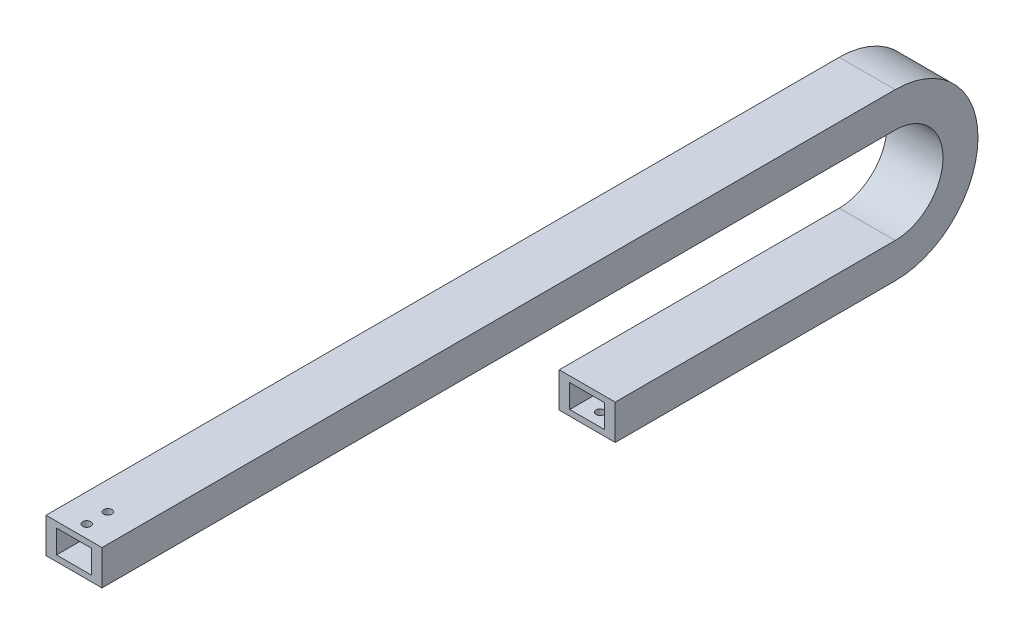
from build123d import *

# Parameters (mm, degrees)
SKETCH_1_W          = 24
SKETCH_1_H          = 15
SKETCH_1_W_2        = 15
SKETCH_1_H_2        = 10
SKETCH_3_R          = 1.75
CUT_EXTRUDE_1_DEPTH = 5
SKETCH_4_R          = 1.75
CUT_EXTRUDE_2_DEPTH = 5


with BuildPart() as part:
    # 扫描1: sweep along a path in 草图2
    with BuildLine(Plane(origin=(0, 0, 0), x_dir=(0, 0, -1), z_dir=(1, 0, 0))) as sweep_1_path:
        Line((0, 0), (120, 0))
        ThreePointArc((120, 0), (148, 28), (120, 56))
        Line((120, 56), (-220, 56))
    # 草图1 → 扫描1 (sweep)
    with BuildSketch(Plane.XY):
        Rectangle(SKETCH_1_W, SKETCH_1_H)
        Rectangle(SKETCH_1_W_2, SKETCH_1_H_2, mode=Mode.SUBTRACT)
    sweep(path=sweep_1_path.line)

    # 草图3 → 切除-拉伸1 (cut)
    with BuildSketch(Plane(origin=(0, 63.5, 0), x_dir=(1, 0, 0), z_dir=(0, 1, 0))):
        with Locations(Location((0, -214.5, 0), (0, 0, 180))):
            Circle(SKETCH_3_R)
        with Locations(Location((0, -205.5, 0), (0, 0, 180))):
            Circle(SKETCH_3_R)
    extrude(amount=-CUT_EXTRUDE_1_DEPTH, mode=Mode.SUBTRACT)

    # 草图4 → 切除-拉伸2 (cut)
    with BuildSketch(Plane.XZ.offset(7.5)):
        with Locations((0, -5.5)):
            Circle(SKETCH_4_R)
        with Locations((0, -14.5)):
            Circle(SKETCH_4_R)
    extrude(amount=-CUT_EXTRUDE_2_DEPTH, mode=Mode.SUBTRACT)


solid = part.part
